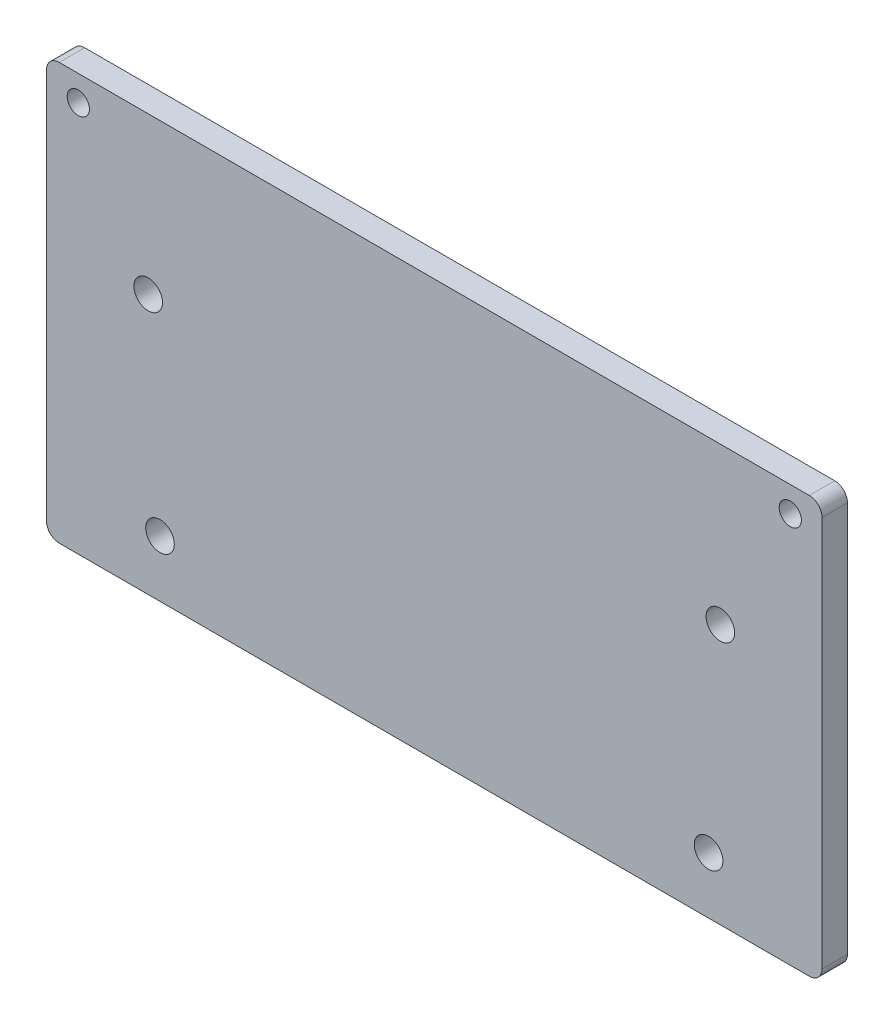
from build123d import *

# Parameters (mm, degrees)
SKETCH_1_W      = 122
SKETCH_1_H      = 65.5
SKETCH_1_R      = 1.75
SKETCH_1_R_2    = 2.25
EXTRUDE_1_DEPTH = 2
FILLET_1_R      = 2


with BuildPart() as part:
    # 草图1 → 凸台-拉伸1 (new, symmetric)
    with BuildSketch(Plane.XY):
        Rectangle(SKETCH_1_W, SKETCH_1_H)
        with Locations((-56, 28.75)):
            Circle(SKETCH_1_R, mode=Mode.SUBTRACT)
        with Locations((-45, 8.15)):
            Circle(SKETCH_1_R_2, mode=Mode.SUBTRACT)
        with Locations((45, 8.15)):
            Circle(SKETCH_1_R_2, mode=Mode.SUBTRACT)
        with Locations(Location((56, 28.75, 0), (0, 0, 180))):
            Circle(SKETCH_1_R, mode=Mode.SUBTRACT)
        with Locations((-43.15, -23.85)):
            Circle(SKETCH_1_R_2, mode=Mode.SUBTRACT)
        with Locations((43.15, -23.85)):
            Circle(SKETCH_1_R_2, mode=Mode.SUBTRACT)
    extrude(amount=EXTRUDE_1_DEPTH, both=True)

    # 圆角1
    fillet_1_edges = [part.edges().sort_by_distance(p)[0] for p in [
        (61, -32.75, 0),
        (-61, -32.75, 0),
        (-61, 32.75, 0),
        (61, 32.75, 0),
    ]]
    fillet(fillet_1_edges, radius=FILLET_1_R)


solid = part.part
